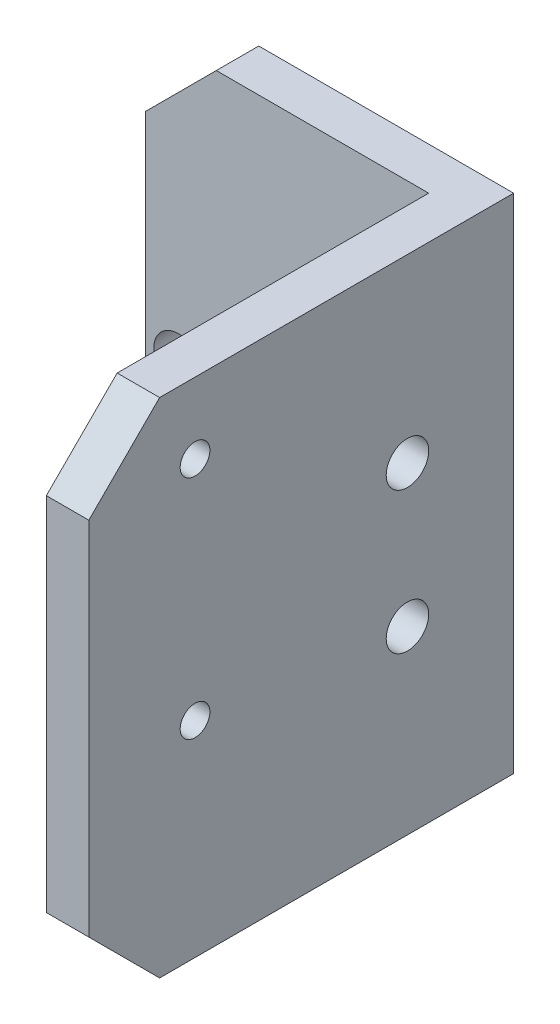
SolidWorks part; units mm, degrees
ref_plane "前视基准面" through (0, 0, 0) normal (0, 0, 1) x (1, 0, 0)
ref_plane "上视基准面" through (0, 0, 0) normal (0, 1, 0) x (1, 0, 0)
ref_plane "右视基准面" through (0, 0, 0) normal (1, 0, 0) x (0, 0, -1)
sketch "草图1" plane through (0, 0, 0) normal (1, 0, 0) x (0, 0, -1)
  line L1 (-30, 35.5) -> (30, 35.5)
  line L2 (-30, 35.5) -> (-30, -35.5)
  line L3 (-30, -35.5) -> (30, -35.5)
  line L4 (30, 35.5) -> (30, -35.5)
  line L5 (-30, 35.5) -> (30, -35.5) construction
  line L6 (-30, -35.5) -> (30, 35.5) construction
  point P0 (0, 0)
  dimension "D1" = 60
  dimension "D2" = 71
extrude "凸台-拉伸1" add sketch "草图1" along normal blind 6
hole_wizard "M5 螺纹孔1" positions "草图2" profile "草图3" tap size "M5" standard "GB" end condition through all
sketch "草图2" plane through (6, 0, 0) normal (1, 0, 0) x (0, 0, -1)
  line L0 (30, 35.5) -> (-30, 35.5) construction
  line L2 (-30, 35.5) -> (-30, -35.5) construction
  point P0 (-15, 25.5)
  point P2 (-15, -6.5)
  dimension "D1" = 32
  dimension "D2" = 10
  dimension "D3" = 15
sketch "草图3" plane through (6, 25.5, 15) normal (0, 1, 0) x (0, 0, -1)
  line L0 (0, 0) -> (0, 6)
  line L1 (0, 6) -> (2.1, 6)
  line L2 (2.1, 6) -> (2.1, 0)
  line L5 (2.1, 0) -> (0, 0)
  line L11 (0, -6.35) -> (0, 107.95) construction
  dimension "通孔螺纹孔钻头直径" = 4.2
  dimension "通孔螺纹孔钻头深度" = 6
cosmetic thread "孔螺蚊线1" parameters "D2"=5
cosmetic thread "孔螺蚊线2" parameters "D2"=5
hole_wizard "Ø6.0 (6) 直径孔1" positions "草图5" profile "草图6" hole size "Ø6.0" standard "GB" end condition through all
sketch "草图5" plane through (0, 0, 0) normal (-1, 0, 0) x (0, 0, 1)
  line L0 (-30, -35.5) -> (-30, 35.5) construction
  line L2 (0, 0) -> (-40.2764, 0) construction
  point P0 (-15, 10)
  point P7 (-15, -10)
  dimension "D1" = 15
  dimension "D3" = 20
sketch "草图6" plane through (0, 10, -15) normal (0, 1, 0) x (0, 0, 1)
  line L0 (0, 0) -> (0, 6)
  line L1 (0, 6) -> (3, 6)
  line L2 (3, 6) -> (3, 0)
  line L5 (3, 0) -> (0, 0)
  line L11 (0, -6.35) -> (0, 107.95) construction
  dimension "通孔孔直径" = 6
  dimension "通孔孔深度" = 6
sketch "草图7" plane through (0, 0, 0) normal (-1, 0, 0) x (0, 0, 1)
  line L0 (30, -35.5) -> (-30, -35.5) construction
  line L1 (-30, 35.5) -> (-24, 35.5)
  line L2 (-30, 35.5) -> (-30, -35.5)
  line L3 (-30, -35.5) -> (-24, -35.5)
  line L4 (-24, 35.5) -> (-24, -35.5)
  dimension "D1" = 6
extrude "凸台-拉伸2" add sketch "草图7" along normal blind 40
hole_wizard "Ø7.0 (7) 直径孔1" positions "草图8" profile "草图9" hole size "Ø7.0" standard "GB"
sketch "草图8" plane through (0, 0, -30) normal (0, 0, -1) x (-1, 0, 0)
  line L0 (0, 0) -> (71.8376, 0) construction
  line L2 (40, 35.5) -> (40, -35.5) construction
  point P0 (20, 10)
  dimension "D1" = 10
  dimension "D2" = 20
sketch "草图9" plane through (-20, 10, -30) normal (1, 0, 0) x (0, 1, 0)
  line L0 (0, 0) -> (0, 17.103)
  line L1 (0, 17.103) -> (3.5, 15)
  line L2 (3.5, 15) -> (3.5, 0)
  line L5 (3.5, 0) -> (0, 0)
  line L10 (0, 17.103) -> (-3.5, 15) construction
  line L11 (0, -6.35) -> (0, 107.95) construction
  dimension "孔直径" = 7
  dimension "孔深度" = 15
  dimension "导头角度" = 118
sketch "草图10" plane through (0, 0, -30) normal (0, 0, -1) x (-1, 0, 0)
  line L2 (20, 10) -> (20, -20.8406) construction
  line L3 (4.6791, -2.8558) -> (20, 10) construction
  line L4 (20, 10) -> (35.3209, -2.8558) construction
  arc A0 (1.998, -5.1055) -> (38.002, -5.1055) centre (20, 10) ccw
  arc A1 (7.3603, -0.606) -> (32.6397, -0.606) centre (20, 10) ccw
  arc A2 (7.3603, -0.606) -> (1.998, -5.1055) centre (4.6791, -2.8558) ccw
  arc A3 (38.002, -5.1055) -> (32.6397, -0.606) centre (35.3209, -2.8558) ccw
  dimension "D1" = 16.5
  dimension "D2" = 23.5
  dimension "D3" = 100
extrude "切除-拉伸1" cut sketch "草图10" against normal through all
chamfer "倒角1" distance 10 angle 45 4 edges at (3, -35.5, 30) (3, 35.5, 30) (-40, -35.5, -27) (-40, 35.5, -27)
